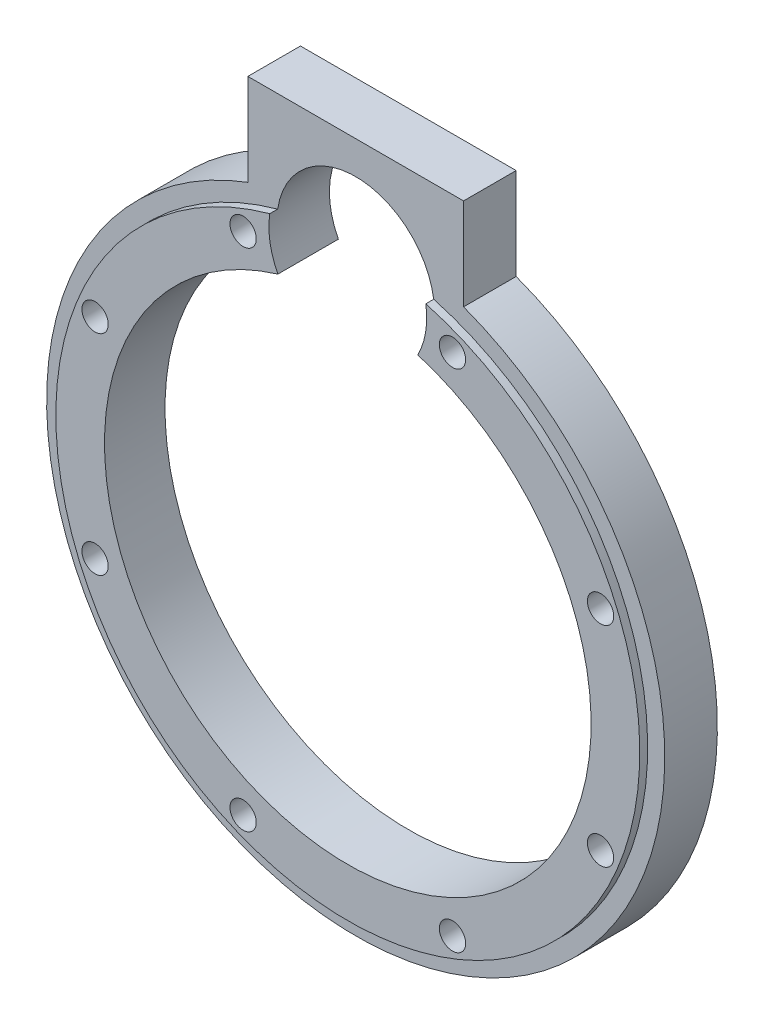
from build123d import *

# Parameters (mm, degrees)
SKETCH_1_R          = 117.5
SKETCH_1_R_2        = 92.5
EXTRUDE_1_DEPTH     = 20
SKETCH_2_W          = 82
SKETCH_2_H          = 52.5
EXTRUDE_2_DEPTH     = 20
SKETCH_7_R          = 111
SKETCH_7_R_2        = 92.5
EXTRUDE_3_DEPTH     = 3
SKETCH_3_R          = 30
CUT_EXTRUDE_1_DEPTH = 189.043213119
HOLE_WIZARD_M8_1_D  = 10


with BuildPart() as part:
    # 草图1 → 凸台-拉伸1 (new body)
    with BuildSketch(Plane.XY):
        Circle(SKETCH_1_R)
        Circle(SKETCH_1_R_2, mode=Mode.SUBTRACT)
    extrude(amount=EXTRUDE_1_DEPTH)

    # 草图2 → 凸台-拉伸2 (add, through all)
    with BuildSketch(Plane.XY.offset(20)):
        with Locations((0, 118.75)):
            Rectangle(SKETCH_2_W, SKETCH_2_H)
    extrude(amount=-EXTRUDE_2_DEPTH)

    # 草图7 → 凸台-拉伸3 (add)
    with BuildSketch(Plane.XY.offset(20)):
        Circle(SKETCH_7_R)
        Circle(SKETCH_7_R_2, mode=Mode.SUBTRACT)
    extrude(amount=EXTRUDE_3_DEPTH)

    # 草图3 → 切除-拉伸1 (cut, through all)
    with BuildSketch(Plane(origin=(0, 0, 0), x_dir=(-1, 0, 0), z_dir=(0, 0, -1))):
        with Locations((0, 102.5)):
            Circle(SKETCH_3_R)
    extrude(amount=-CUT_EXTRUDE_1_DEPTH, mode=Mode.SUBTRACT)

    # M8 间隙孔1 (through all)
    with Locations(Plane(origin=(0, 0, 0), x_dir=(-1, 0, 0), z_dir=(0, 0, -1))):
        with Locations((-39.799076966, 96.083471381), (-96.083471381, 39.799076966), (-96.083471381, -39.799076966), (-39.799076966, -96.083471381), (39.799076966, -96.083471381), (96.083471381, -39.799076966), (96.083471381, 39.799076966), (39.799076966, 96.083471381)):
            Hole(HOLE_WIZARD_M8_1_D / 2)


solid = part.part
